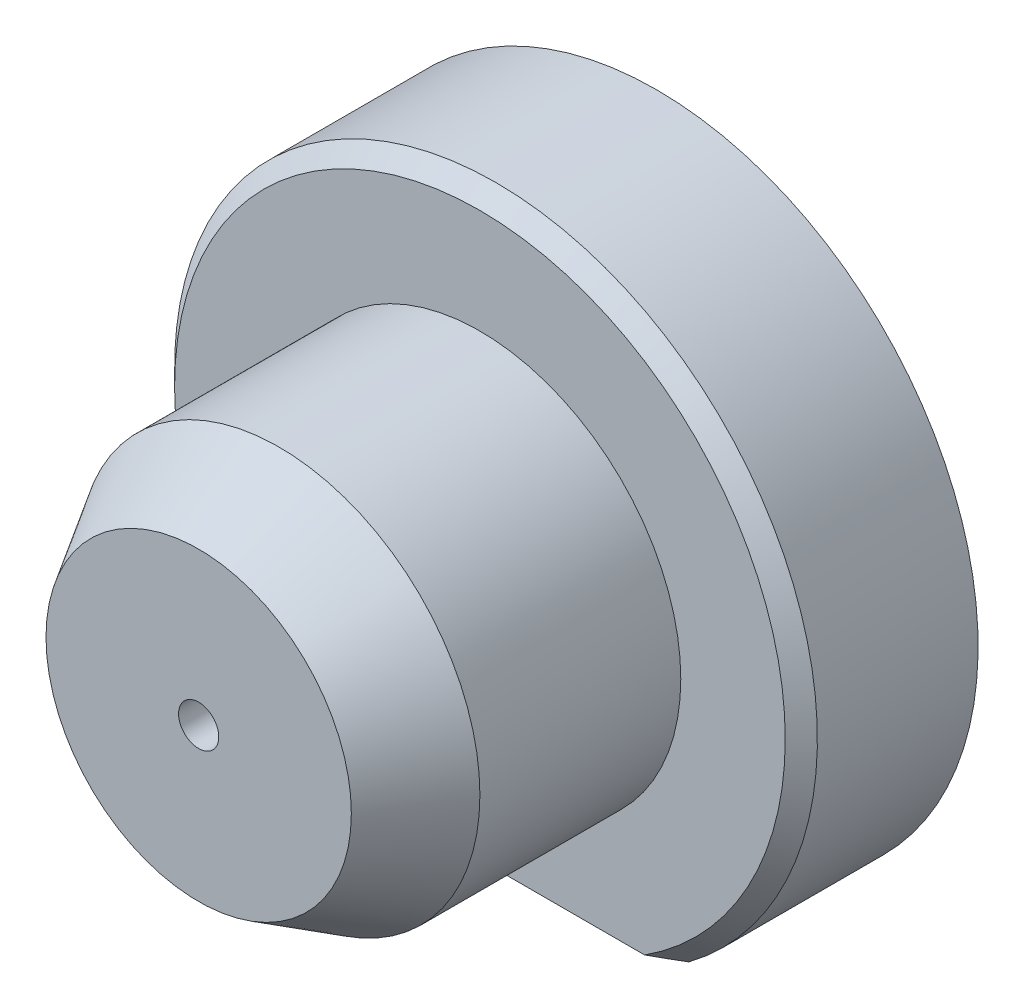
from build123d import *

# Parameters (mm, degrees)
SKETCH1_R           = 25
BOSS_EXTRUDE1_DEPTH = 35
CHAMFER1_SIZE       = 10
CHAMFER1_SIZE2      = 6
SKETCH2_R           = 40
BOSS_EXTRUDE2_DEPTH = 22
SKETCH3_W           = 90
SKETCH3_H           = 30
CUT_EXTRUDE1_DEPTH  = 30
CHAMFER2_SIZE       = 2
M6_TAPPED_HOLE1_D   = 5


with BuildPart() as part:
    # Sketch1 → Boss-Extrude1 (new body)
    with BuildSketch(Plane.XY):
        Circle(SKETCH1_R)
    extrude(amount=BOSS_EXTRUDE1_DEPTH)

    # Chamfer1
    chamfer1_edges = [part.edges().sort_by_distance(p)[0] for p in [
        (-25, 0, 35),
    ]]
    chamfer1_side = [part.faces().sort_by_distance(p)[0] for p in [
        (-25, 0, 17.5),
    ]]
    chamfer(chamfer1_edges, length=CHAMFER1_SIZE, length2=CHAMFER1_SIZE2, reference=chamfer1_side[0])

    # Sketch2 → Boss-Extrude2 (add)
    with BuildSketch(Plane(origin=(0, 0, 0), x_dir=(-1, 0, 0), z_dir=(0, 0, -1))):
        Circle(SKETCH2_R)
    extrude(amount=BOSS_EXTRUDE2_DEPTH)

    # Sketch3 → Cut-Extrude1 (cut, symmetric)
    with BuildSketch(Plane(origin=(0, 0, 0), x_dir=(0, 0, -1), z_dir=(1, 0, 0))):
        with Locations((-23, -47)):
            Rectangle(SKETCH3_W, SKETCH3_H)
    extrude(amount=CUT_EXTRUDE1_DEPTH, both=True, mode=Mode.SUBTRACT)

    # Chamfer2
    chamfer2_edges = [part.edges().sort_by_distance(p)[0] for p in [
        (0, 40, 0),
    ]]
    chamfer(chamfer2_edges, length=CHAMFER2_SIZE)

    # M6 Tapped Hole1 (through all)
    with Locations(Plane(origin=(0, 0, -22), x_dir=(-1, 0, 0), z_dir=(0, 0, -1))):
        with Locations((0, 0)):
            Hole(M6_TAPPED_HOLE1_D / 2)


solid = part.part
